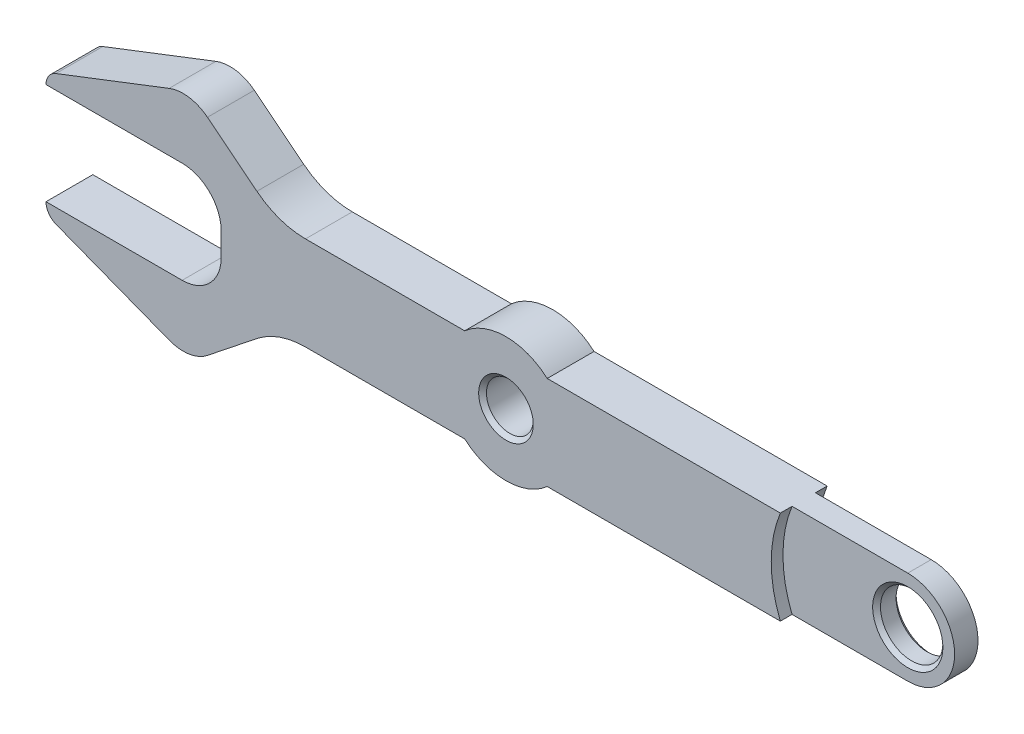
SolidWorks part; units mm, degrees
ref_plane "Front Plane" through (0, 0, 0) normal (0, 0, 1) x (1, 0, 0)
ref_plane "Top Plane" through (0, 0, 0) normal (0, 1, 0) x (1, 0, 0)
ref_plane "Right Plane" through (0, 0, 0) normal (1, 0, 0) x (0, 0, -1)
other "Configuration Table"
sketch "Sketch1" plane through (0, 0, 0) normal (0, 0, 1) x (1, 0, 0)
  line L0 (-98.3471, 0) -> (90.5785, 0) construction
  line L3 (50, 6) -> (5.2915, 6)
  line L4 (-36.5, -1.5) -> (-36.5, 1.5)
  line L9 (-41.5, 6.5) -> (-62.5, 6.5) construction
  line L10 (-5.2915, 6) -> (-29.1854, 6)
  line L11 (-29.1854, 6) -> (-38.2579, 13.2165)
  line L12 (-43.1724, 13.9675) -> (-62.5, 6.5) construction
  line L13 (-58.9506, 6.5) -> (-41.5, 6.5)
  line L14 (-43.1724, 13.9675) -> (-57.6714, 8.3656)
  line L15 (-43.1724, -13.9675) -> (-62.5, -6.5) construction
  line L16 (-41.5, -6.5) -> (-62.5, -6.5) construction
  line L17 (-43.1724, -13.9675) -> (-57.6714, -8.3656)
  line L18 (-58.9506, -6.5) -> (-41.5, -6.5)
  line L19 (-29.1854, -6) -> (-38.2579, -13.2165)
  line L20 (-5.2915, -6) -> (-29.1854, -6)
  line L21 (50, -6) -> (5.2915, -6)
  arc A2 (5.2915, 6) -> (-5.2915, 6) centre (0, 0) ccw
  arc A3 (50, -6) -> (50, 6) centre (50, 0) ccw
  arc A4 (-36.5, 1.5) -> (-41.5, 6.5) centre (-41.5, 1.5) ccw
  arc A5 (-38.2579, 13.2165) -> (-43.1724, 13.9675) centre (-41.3704, 9.3035) ccw
  arc A6 (-58.9506, 6.5) -> (-57.6714, 8.3656) centre (-56.9506, 6.5) cw
  arc A7 (-58.9506, -6.5) -> (-57.6714, -8.3656) centre (-56.9506, -6.5) ccw
  arc A8 (-38.2579, -13.2165) -> (-43.1724, -13.9675) centre (-41.3704, -9.3035) cw
  arc A9 (-36.5, -1.5) -> (-41.5, -6.5) centre (-41.5, -1.5) cw
  arc A10 (5.2915, -6) -> (-5.2915, -6) centre (0, 0) cw
  point P9 (-40.5, -15)
  point P19 (-36.5, 6.5)
  point P22 (-40.5, 15)
  point P36 (-36.5, 0)
  point P37 (-36.5, -6.5)
  dimension "D2" = 12
  dimension "D3" = 16
  dimension "D10" = 5
  dimension "D11" = 2
  dimension "D1" = 50
  dimension "D4" = 6.5
  dimension "D5" = 26
  dimension "D6" = 112.5
  dimension "D7" = 38.5
  dimension "D8" = 30
  dimension "D9" = 22
extrude "Boss-Extrude1" add sketch "Sketch1" along normal mid plane 6
sketch "Sketch3" plane through (0, 0, 3) normal (0, 0, 1) x (1, 0, 0)
  circle A0 centre (50, 0) radius 16
  dimension "D1" = 32
extrude "Cut-Extrude1" cut sketch "Sketch3" against normal blind 1.5
mirror "Mirror1" about plane through (0, 0, 0) normal (0, 0, 1) of "Cut-Extrude1"
sketch "Sketch4" plane through (0, 0, 1.5) normal (0, 0, 1) x (1, 0, 0)
  circle A0 centre (50, 0) radius 4
  circle A1 centre (0, 0) radius 3
  dimension "D1" = 6
  dimension "D2" = 8
extrude "Cut-Extrude2" cut sketch "Sketch4" against normal through all both and the other way through all
chamfer "Chamfer1" distance 0.5 angle 45 4 edges at (46, 0, -1.5) (54, 0, 1.5) (3, 0, 3) (3, 0, -3)
fillet "Fillet1" radius 10 2 edges at (-29.1854, -6, 0) (-29.1854, 6, 0)
